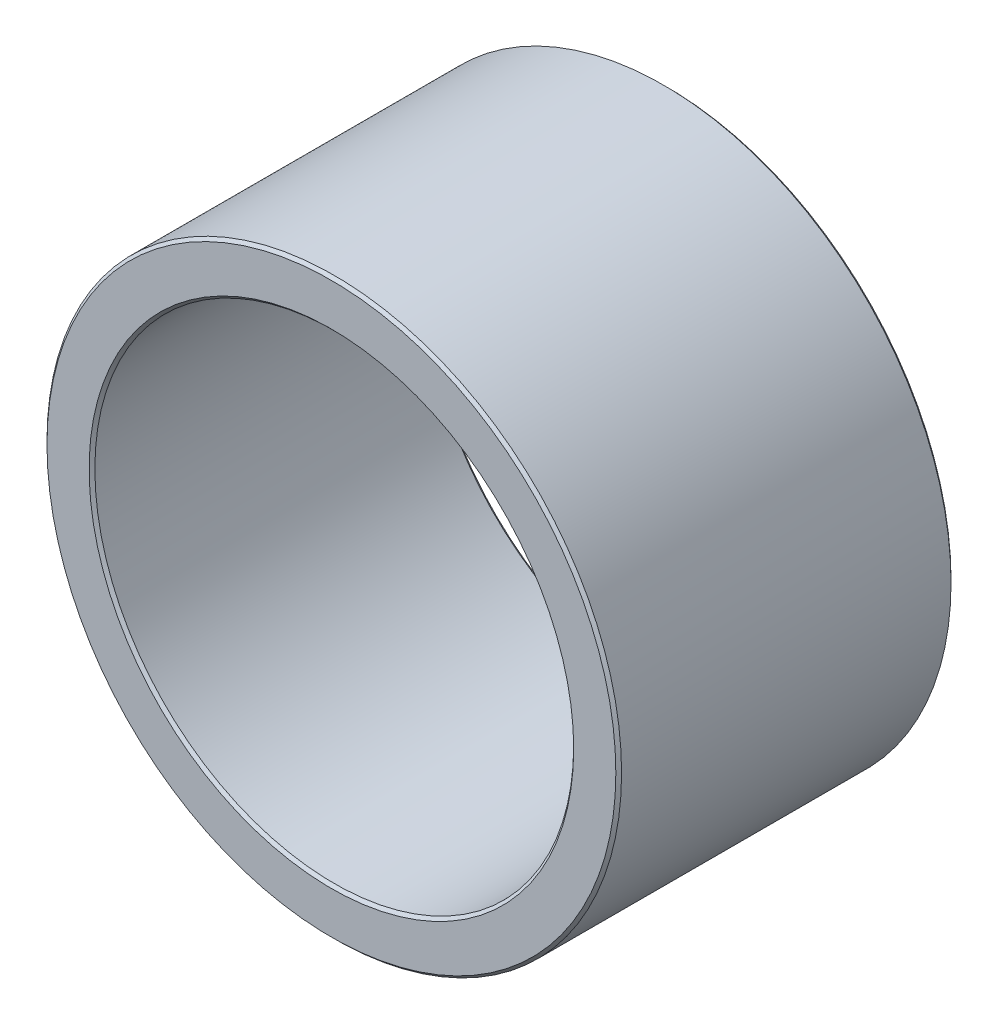
from build123d import *

# Parameters (mm, degrees)
SKETCH1_R           = 30
SKETCH1_R_2         = 25
BOSS_EXTRUDE1_DEPTH = 35
CHAMFER1_SIZE       = 0.3


with BuildPart() as part:
    # Sketch1 → Boss-Extrude1 (new body)
    with BuildSketch(Plane.XY):
        Circle(SKETCH1_R)
        Circle(SKETCH1_R_2, mode=Mode.SUBTRACT)
    extrude(amount=BOSS_EXTRUDE1_DEPTH)

    # Chamfer1
    chamfer1_edges = [part.edges().sort_by_distance(p)[0] for p in [
        (-30, 0, 0),
        (-30, 0, 35),
        (-25, 0, 0),
        (-25, 0, 35),
    ]]
    chamfer(chamfer1_edges, length=CHAMFER1_SIZE)


solid = part.part
